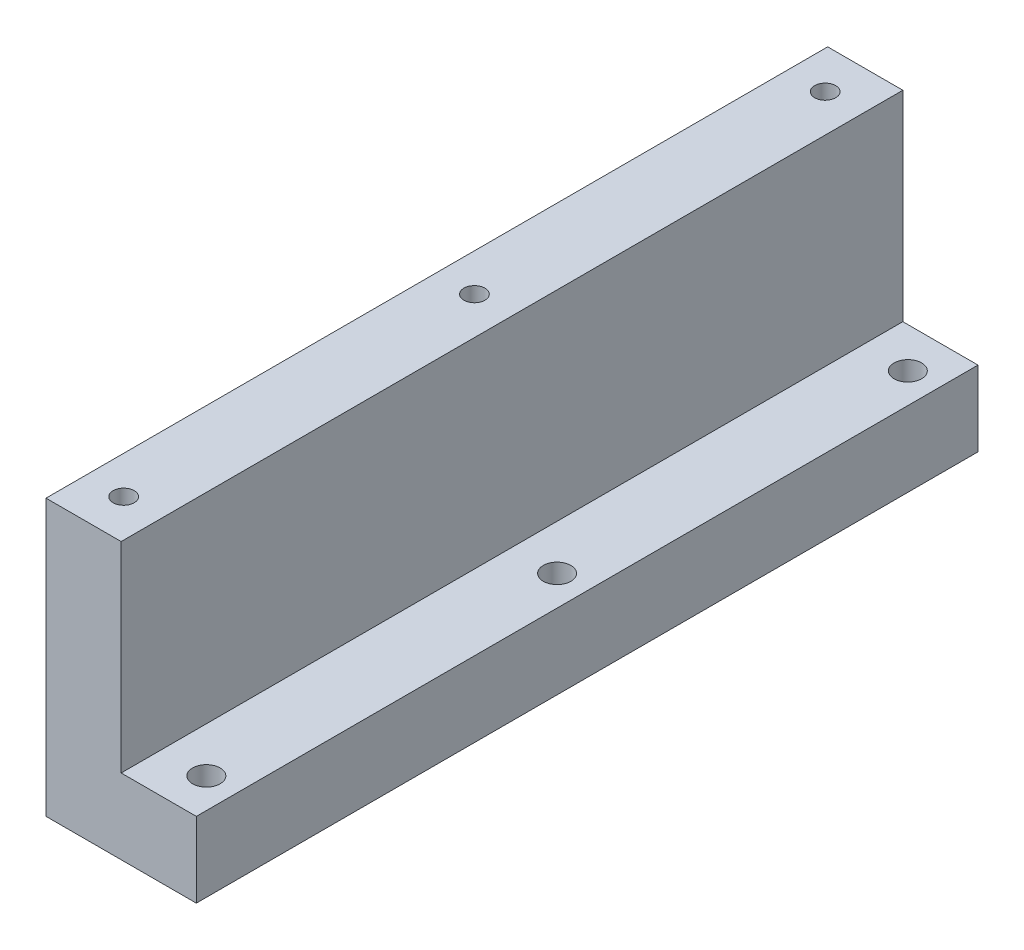
SolidWorks part; units mm, degrees
material "45#"
ref_plane "Front Plane" through (0, 0, 0) normal (0, 0, 1) x (1, 0, 0)
ref_plane "Top Plane" through (0, 0, 0) normal (0, 1, 0) x (1, 0, 0)
ref_plane "Right Plane" through (0, 0, 0) normal (1, 0, 0) x (0, 0, -1)
sketch "Sketch1" plane through (0, 0, 0) normal (0, 0, 1) x (1, 0, 0)
  line L0 (0, 55) -> (0, 0)
  line L1 (0, 0) -> (30, 0)
  line L2 (30, 0) -> (30, 15)
  line L3 (30, 15) -> (15, 15)
  line L4 (15, 15) -> (15, 55)
  line L5 (15, 55) -> (0, 55)
  dimension "D1" = 15
  dimension "D2" = 30
  dimension "D3" = 55
extrude "Extrude1" add sketch "Sketch1" along normal mid plane 156
hole_wizard "M5 Tapped Hole1" positions "3D Sketch1" profile "Sketch2" tap size "M5" standard "ISO"
sketch3d "3D Sketch1"
  line L0 (0, 55, 0) -> (15, 55, 0) construction
  line L1 (0, 55, 78) -> (0, 55, -78) construction
  line L2 (15, 55, 78) -> (15, 55, -78) construction
  line L4 (7.5, 55, 0) -> (7.5, 55, -70) construction
  line L6 (7.5, 55, 0) -> (7.5, 55, 70) construction
  point P0 (7.5, 55, 0)
  point P2 (7.5, 55, -70)
  point P4 (7.5, 55, 70)
  dimension "D1" = 140
sketch "Sketch2" plane through (7.5, 55, 0) normal (1, 0, 0) x (0, 0, 1)
  line L0 (0, 0) -> (0, 15.6618)
  line L1 (0, 15.6618) -> (2.1, 14.4)
  line L2 (2.1, 14.4) -> (2.1, 0)
  line L5 (2.1, 0) -> (0, 0)
  line L10 (0, 15.6618) -> (-2.1, 14.4) construction
  line L11 (0, -6.35) -> (0, 107.95) construction
  dimension "螺孔鑽直徑" = 4.2
  dimension "螺孔鑽深度" = 14.4
  dimension "導頭角度" = 118
cosmetic thread "Cosmetic Thread1" parameters "D1"=12, "D2"=5
cosmetic thread "Cosmetic Thread2" parameters "D1"=12, "D2"=5
cosmetic thread "Cosmetic Thread3" parameters "D1"=12, "D2"=5
sketch "Sketch3" plane through (0, 15, 0) normal (0, 1, 0) x (1, 0, 0)
  line L0 (30, 0) -> (-12.702, 0) construction
  line L1 (30, -78) -> (30, 78) construction
  line L2 (24, 70) -> (24, 0) construction
  circle A0 centre (24, 0) radius 2.75
  circle A1 centre (24, 70) radius 2.75
  circle A2 centre (24, -70) radius 2.75
  dimension "D1" = 5.5
  dimension "D3" = 140
  dimension "D2" = 6
extrude "Cut-Extrude1" cut sketch "Sketch3" against normal through all
